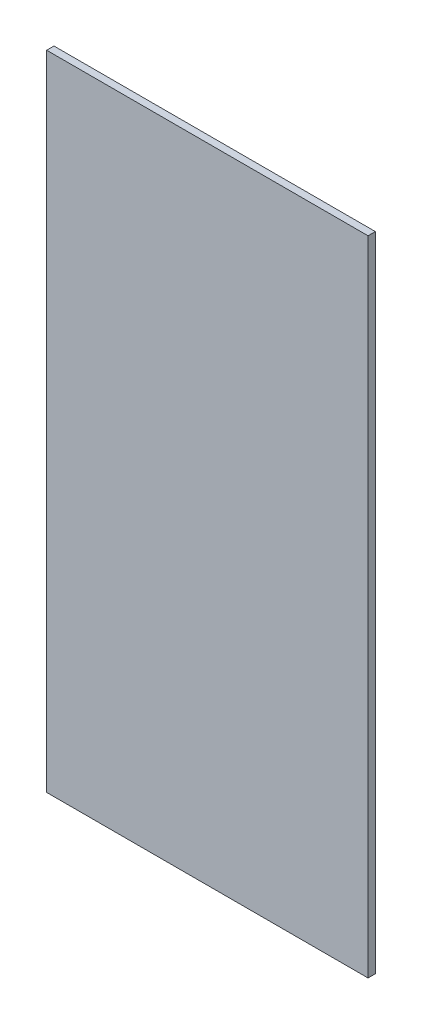
SolidWorks part; units mm, degrees
material "标准件"
ref_plane "前视基准面" through (0, 0, 0) normal (0, 0, 1) x (1, 0, 0)
ref_plane "上视基准面" through (0, 0, 0) normal (0, 1, 0) x (1, 0, 0)
ref_plane "右视基准面" through (0, 0, 0) normal (1, 0, 0) x (0, 0, -1)
sketch "草图1" plane through (0, 0, 0) normal (0, 0, 1) x (1, 0, 0)
  line L1 (-22, -44) -> (22, -44)
  line L2 (-22, -44) -> (-22, 44)
  line L3 (-22, 44) -> (22, 44)
  line L4 (22, -44) -> (22, 44)
  line L5 (-22, -44) -> (22, 44) construction
  line L6 (-22, 44) -> (22, -44) construction
  point P0 (0, 0)
  dimension "D1" = 44
  dimension "D2" = 88
extrude "凸台-拉伸1" add sketch "草图1" along normal mid plane 1
